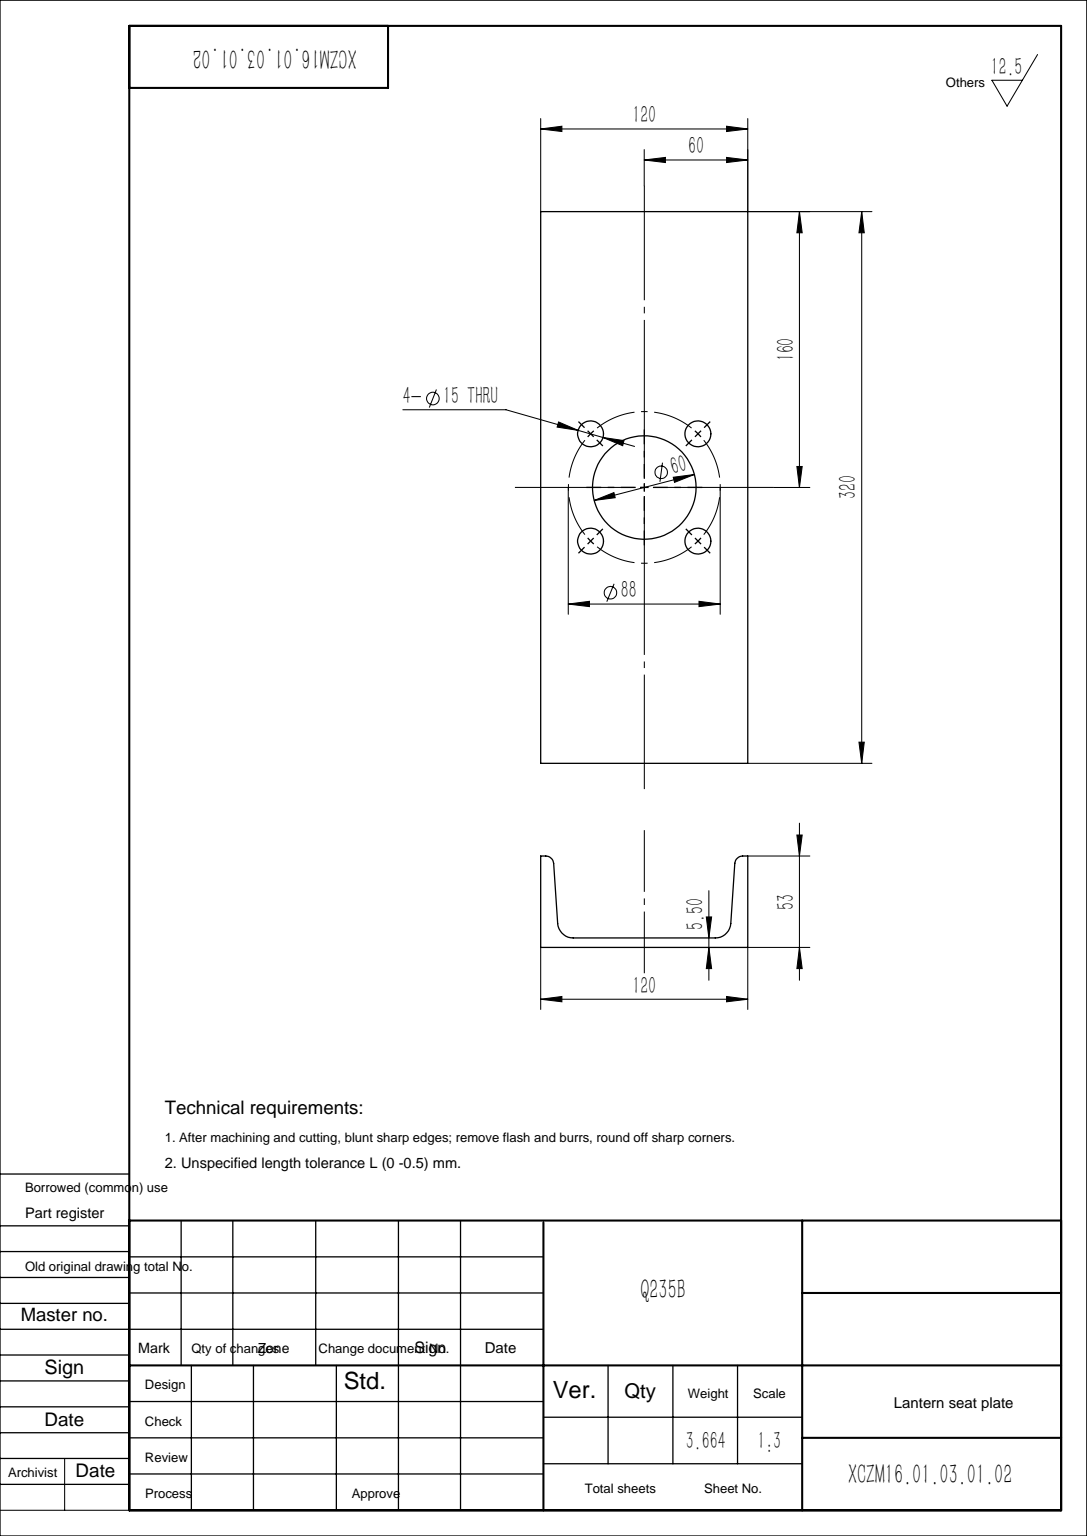
from build123d import *

# Parameters (mm, degrees)
MEMBER_12_1_DEPTH   = 320
SKETCH_5_R          = 30
SKETCH_5_R_2        = 7.5
CUT_EXTRUDE_1_DEPTH = 10


with BuildPart() as part:
    # Sketch1 → Member 12_1 (new body)
    with BuildSketch(Plane.ZX):
        with BuildLine():
            Line((0, 0), (0, -120))
            Line((0, -120), (-53, -120))
            Line((-53, -120), (-53, -117.0157841))
            ThreePointArc((-53, -117.0157841), (-51.788791155, -113.944326346), (-48.807176562, -112.526280502))
            Line((-48.807176562, -112.526280502), (-13.885646876, -110.136912681))
            ThreePointArc((-13.885646876, -110.136912681), (-7.922417689, -107.300820993), (-5.5, -101.157905484))
            Line((-5.5, -101.157905484), (-5.5, -18.842094516))
            ThreePointArc((-5.5, -18.842094516), (-7.922417689, -12.699179007), (-13.885646876, -9.863087319))
            Line((-13.885646876, -9.863087319), (-48.807176562, -7.473719498))
            ThreePointArc((-48.807176562, -7.473719498), (-51.788791155, -6.055673654), (-53, -2.9842159))
            Line((-53, -2.9842159), (-53, 0))
            Line((-53, 0), (0, 0))
        make_face()
    extrude(amount=MEMBER_12_1_DEPTH)

    # 草图5 → 切除-拉伸1 (cut)
    with BuildSketch(Plane.XY):
        with Locations((-60, 160)):
            Circle(SKETCH_5_R)
        with Locations((-91.112698372, 191.112698372)):
            Circle(SKETCH_5_R_2)
        with Locations((-28.887301628, 191.112698372)):
            Circle(SKETCH_5_R_2)
        with Locations((-28.887301628, 128.887301628)):
            Circle(SKETCH_5_R_2)
        with Locations((-91.112698372, 128.887301628)):
            Circle(SKETCH_5_R_2)
    extrude(amount=-CUT_EXTRUDE_1_DEPTH, mode=Mode.SUBTRACT)


solid = part.part
